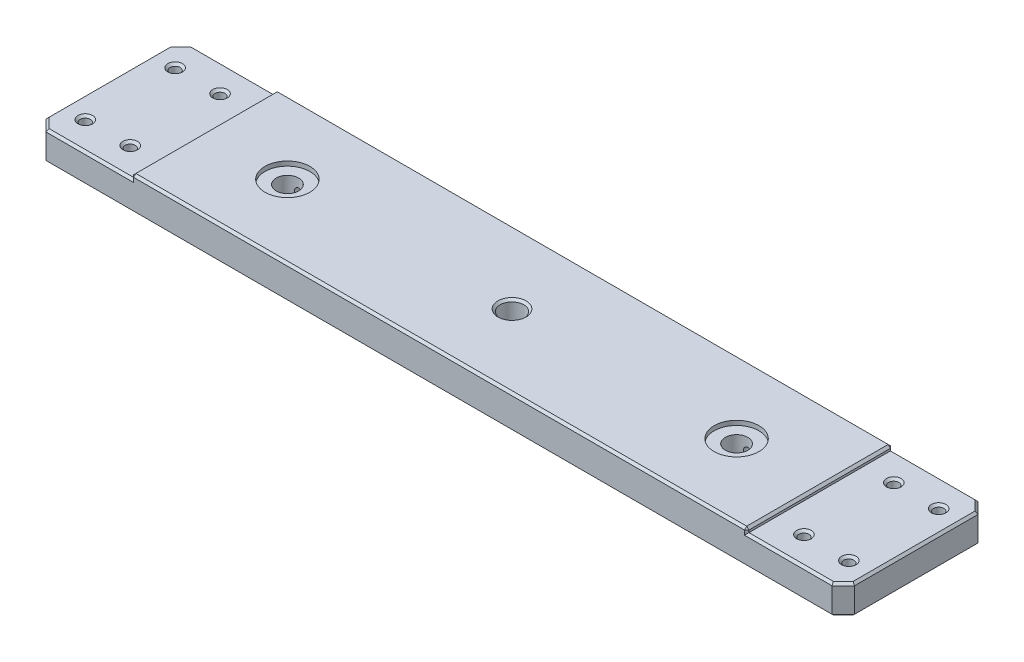
from build123d import *

# Parameters (mm, degrees)
SKETCH1_W                                          = 360
SKETCH1_H                                          = 65
BOSS_EXTRUDE1_DEPTH                                = 15
SKETCH2_W                                          = 43
SKETCH2_H                                          = 65
CUT_EXTRUDE1_DEPTH                                 = 2
HOLE_SIZE_BASED_ON_SOCKET_HEAD_CAP_SCR_D           = 4.5
HOLE_SIZE_BASED_ON_SOCKET_HEAD_CAP_SCR_CBORE_D     = 8
HOLE_SIZE_BASED_ON_SOCKET_HEAD_CAP_SCR_CBORE_DEPTH = 4.6
M12X1_5_TAPPED_HOLE1_D                             = 10.5
CHAMFER1_SIZE                                      = 5
CHAMFER2_SIZE                                      = 1
SKETCH7_R                                          = 5
CUT_EXTRUDE2_DEPTH                                 = 184.524521522
M4_TAPPED_HOLE1_REACH                              = 193.964
M4_TAPPED_HOLE1_BORE_R                             = 1.65
SKETCH10_R                                         = 10
CUT_EXTRUDE3_DEPTH                                 = 2


with BuildPart() as part:
    # Sketch1 → Boss-Extrude1 (new body)
    with BuildSketch(Plane(origin=(0, 0, 0), x_dir=(1, 0, 0), z_dir=(0, 1, 0))):
        Rectangle(SKETCH1_W, SKETCH1_H)
    extrude(amount=BOSS_EXTRUDE1_DEPTH)

    # Sketch2 → Cut-Extrude1 (cut)
    with BuildSketch(Plane(origin=(0, 15, 0), x_dir=(1, 0, 0), z_dir=(0, 1, 0))):
        with Locations((-158.5, 0)):
            Rectangle(SKETCH2_W, SKETCH2_H)
        with Locations((158.5, 0)):
            Rectangle(SKETCH2_W, SKETCH2_H)
    extrude(amount=-CUT_EXTRUDE1_DEPTH, mode=Mode.SUBTRACT)

    # Hole size (%based on) socket head cap screw type 1 (through all)
    with Locations(Plane(origin=(0, 0, 0), x_dir=(-1, 0, 0), z_dir=(0, -1, 0))):
        with Locations((170, -20), (150, -20), (170, 20), (150, 20), (-150, 20), (-170, 20), (-150, -20), (-170, -20)):
            CounterBoreHole(HOLE_SIZE_BASED_ON_SOCKET_HEAD_CAP_SCR_D / 2, HOLE_SIZE_BASED_ON_SOCKET_HEAD_CAP_SCR_CBORE_D / 2, HOLE_SIZE_BASED_ON_SOCKET_HEAD_CAP_SCR_CBORE_DEPTH)

    # M12x1.5 Tapped Hole1 (through all)
    with Locations(Plane(origin=(0, 0, 0), x_dir=(-1, 0, 0), z_dir=(0, -1, 0))):
        with Locations((0, 0)):
            Hole(M12X1_5_TAPPED_HOLE1_D / 2)

    # Chamfer1
    chamfer1_edges = [part.edges().sort_by_distance(p)[0] for p in [
        (180, 6.5, 32.5),
        (-180, 6.5, 32.5),
        (-180, 6.5, -32.5),
        (180, 6.5, -32.5),
    ]]
    chamfer(chamfer1_edges, length=CHAMFER1_SIZE)

    # Chamfer2
    chamfer2_edges = [part.edges().sort_by_distance(p)[0] for p in [
        (-5.25, 0, 0),
        (-5.25, 15, 0),
        (-156, 13, 32.5),
        (0, 0, 32.5),
        (180, 0, 0),
        (-180, 0, 0),
        (0, 0, -32.5),
        (177.5, 0, -30),
        (177.5, 0, 30),
        (-177.5, 0, -30),
        (-177.5, 0, 30),
        (-180, 13, 0),
        (-177.5, 13, -30),
        (0, 15, -32.5),
        (-177.5, 13, 30),
        (156, 13, -32.5),
        (180, 13, 0),
        (177.5, 13, -30),
        (177.5, 13, 30),
        (0, 15, 32.5),
        (-156, 13, -32.5),
        (-137, 14, -32.5),
        (-137, 14, 32.5),
        (-137, 15, 0),
        (137, 14, -32.5),
        (156, 13, 32.5),
        (137, 14, 32.5),
        (137, 15, 0),
        (167.75, 13, 20),
        (174, 0, 20),
        (147.75, 13, 20),
        (154, 0, 20),
        (167.75, 13, -20),
        (174, 0, -20),
        (147.75, 13, -20),
        (154, 0, -20),
        (-152.25, 13, -20),
        (-146, 0, -20),
        (-172.25, 13, -20),
        (-166, 0, -20),
        (-152.25, 13, 20),
        (-146, 0, 20),
        (-172.25, 13, 20),
        (-166, 0, 20),
    ]]
    chamfer(chamfer2_edges, length=CHAMFER2_SIZE)

    # Sketch7 → Cut-Extrude2 (cut, through all)
    with BuildSketch(Plane(origin=(0, 15, 0), x_dir=(1, 0, 0), z_dir=(0, 1, 0))):
        with Locations(Location((-100, 0, 0), (0, 0, 270))):
            Circle(SKETCH7_R)
        with Locations(Location((100, 0, 0), (0, 0, 90))):
            Circle(SKETCH7_R)
    extrude(amount=-CUT_EXTRUDE2_DEPTH, mode=Mode.SUBTRACT)

    # M4 Tapped Hole1 bore → M4 Tapped Hole1 (cut, up to next)
    with BuildSketch(Plane(origin=(0, 0, -32.5), x_dir=(-1, 0, 0), z_dir=(0, 0, -1)), mode=Mode.PRIVATE) as m4_tapped_hole1_sk1:
        with Locations((-100, 7.5)):
            Circle(M4_TAPPED_HOLE1_BORE_R)
    m4_tapped_hole1_tool1 = extrude(m4_tapped_hole1_sk1.sketch, amount=-M4_TAPPED_HOLE1_REACH, mode=Mode.PRIVATE) & part.part
    # M4 Tapped Hole1 bore → M4 Tapped Hole1 (cut, up to next)
    with BuildSketch(Plane(origin=(0, 0, -32.5), x_dir=(-1, 0, 0), z_dir=(0, 0, -1)), mode=Mode.PRIVATE) as m4_tapped_hole1_sk2:
        with Locations((100, 7.5)):
            Circle(M4_TAPPED_HOLE1_BORE_R)
    m4_tapped_hole1_tool2 = extrude(m4_tapped_hole1_sk2.sketch, amount=-M4_TAPPED_HOLE1_REACH, mode=Mode.PRIVATE) & part.part
    add(m4_tapped_hole1_tool1.solids().sort_by_distance((100, 7.5, -32.5))[0], mode=Mode.SUBTRACT)
    add(m4_tapped_hole1_tool2.solids().sort_by_distance((-100, 7.5, -32.5))[0], mode=Mode.SUBTRACT)

    # Sketch10 → Cut-Extrude3 (cut)
    with BuildSketch(Plane(origin=(0, 15, 0), x_dir=(1, 0, 0), z_dir=(0, 1, 0))):
        with Locations(Location((-100, 0, 0), (0, 0, 270))):
            Circle(SKETCH10_R)
        with Locations(Location((100, 0, 0), (0, 0, 270))):
            Circle(SKETCH10_R)
    extrude(amount=-CUT_EXTRUDE3_DEPTH, mode=Mode.SUBTRACT)


solid = part.part
